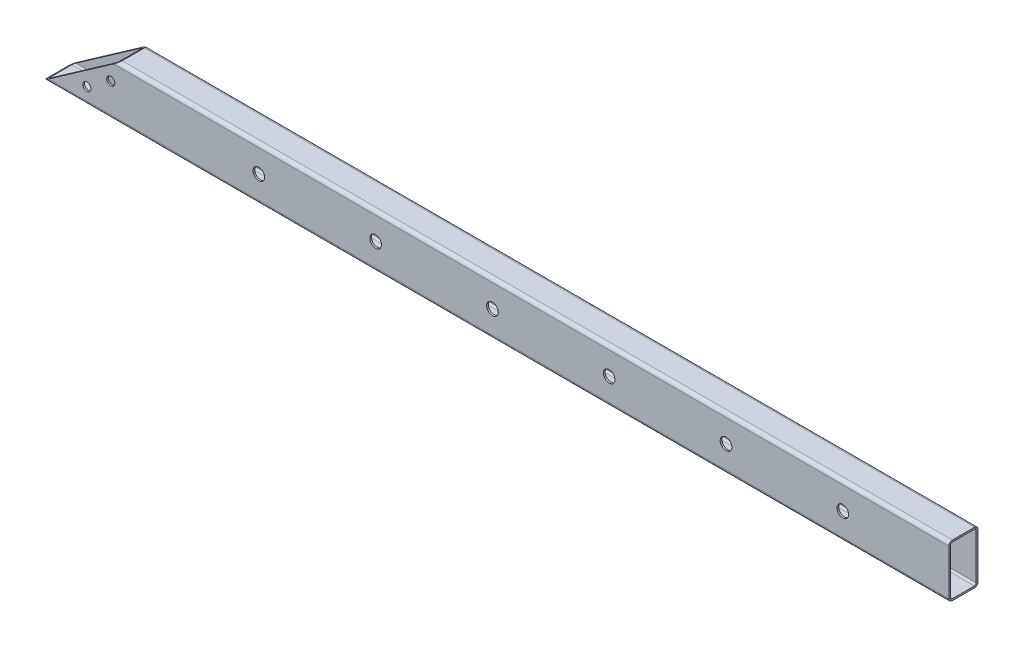
from build123d import *

# Parameters (mm, degrees)
GB_T6728_2002_90_X_50_X_4_1_DEPTH = 1550
HOLE_WIZARD_20_0_20_1_D           = 20
PATTERN_LINEAR_1_COUNT            = 6
PATTERN_LINEAR_1_PITCH            = 200
HOLE_WIZARD_14_0_14_2_D           = 14


with BuildPart() as part:
    # Sketch11 → 冷弯空心矩管gb∕t6728-2002 90 X 50 X 4(1) (new body)
    with BuildSketch(Plane(origin=(0, 0, 0), x_dir=(0, 0, 1), z_dir=(1, 0, 0))):
        with BuildLine():
            Line((-19, -45), (19, -45))
            ThreePointArc((19, -45), (23.242640687, -43.242640687), (25, -39))
            Line((25, -39), (25, 39))
            ThreePointArc((25, 39), (23.242640687, 43.242640687), (19, 45))
            Line((19, 45), (-19, 45))
            ThreePointArc((-19, 45), (-23.242640687, 43.242640687), (-25, 39))
            Line((-25, 39), (-25, -39))
            ThreePointArc((-25, -39), (-23.242640687, -43.242640687), (-19, -45))
        make_face()
        with BuildLine():
            Line((-19, -42), (19, -42))
            ThreePointArc((19, -42), (21.121320344, -41.121320344), (22, -39))
            Line((22, -39), (22, 39))
            ThreePointArc((22, 39), (21.121320344, 41.121320344), (19, 42))
            Line((19, 42), (-19, 42))
            ThreePointArc((-19, 42), (-21.121320344, 41.121320344), (-22, 39))
            Line((-22, 39), (-22, -39))
            ThreePointArc((-22, -39), (-21.121320344, -41.121320344), (-19, -42))
        make_face(mode=Mode.SUBTRACT)
    extrude(amount=GB_T6728_2002_90_X_50_X_4_1_DEPTH)

    # Split Bodies 1
    split(bisect_by=Plane(origin=(21.143083968, -30.195453225, 0), x_dir=(-0.819152044288993, -0.5735764363510444, 0), z_dir=(0.5735764363510444, -0.819152044288993, -2.99158375078423e-15)), keep=Keep.TOP)

    # Ø20.0 (20) 直径孔1 (through all)
    with Locations(Plane.XY.offset(25)):
        with Locations((368.533320607, 0)):
            hole_wizard_20_0_20_1 = Hole(HOLE_WIZARD_20_0_20_1_D / 2)

    # 阵列(线性)1: Ø20.0 (20) 直径孔1 ×6
    with Locations(*[(i * PATTERN_LINEAR_1_PITCH, 0, 0) for i in range(1, PATTERN_LINEAR_1_COUNT)]):
        add(hole_wizard_20_0_20_1, mode=Mode.SUBTRACT)

    # Ø14.0 (14) 直径孔2 (through all)
    with Locations(Plane.XY.offset(25)):
        with Locations((115.028466248, 11.128307401), (74.070864034, -17.550514417)):
            Hole(HOLE_WIZARD_14_0_14_2_D / 2)


solid = part.part
